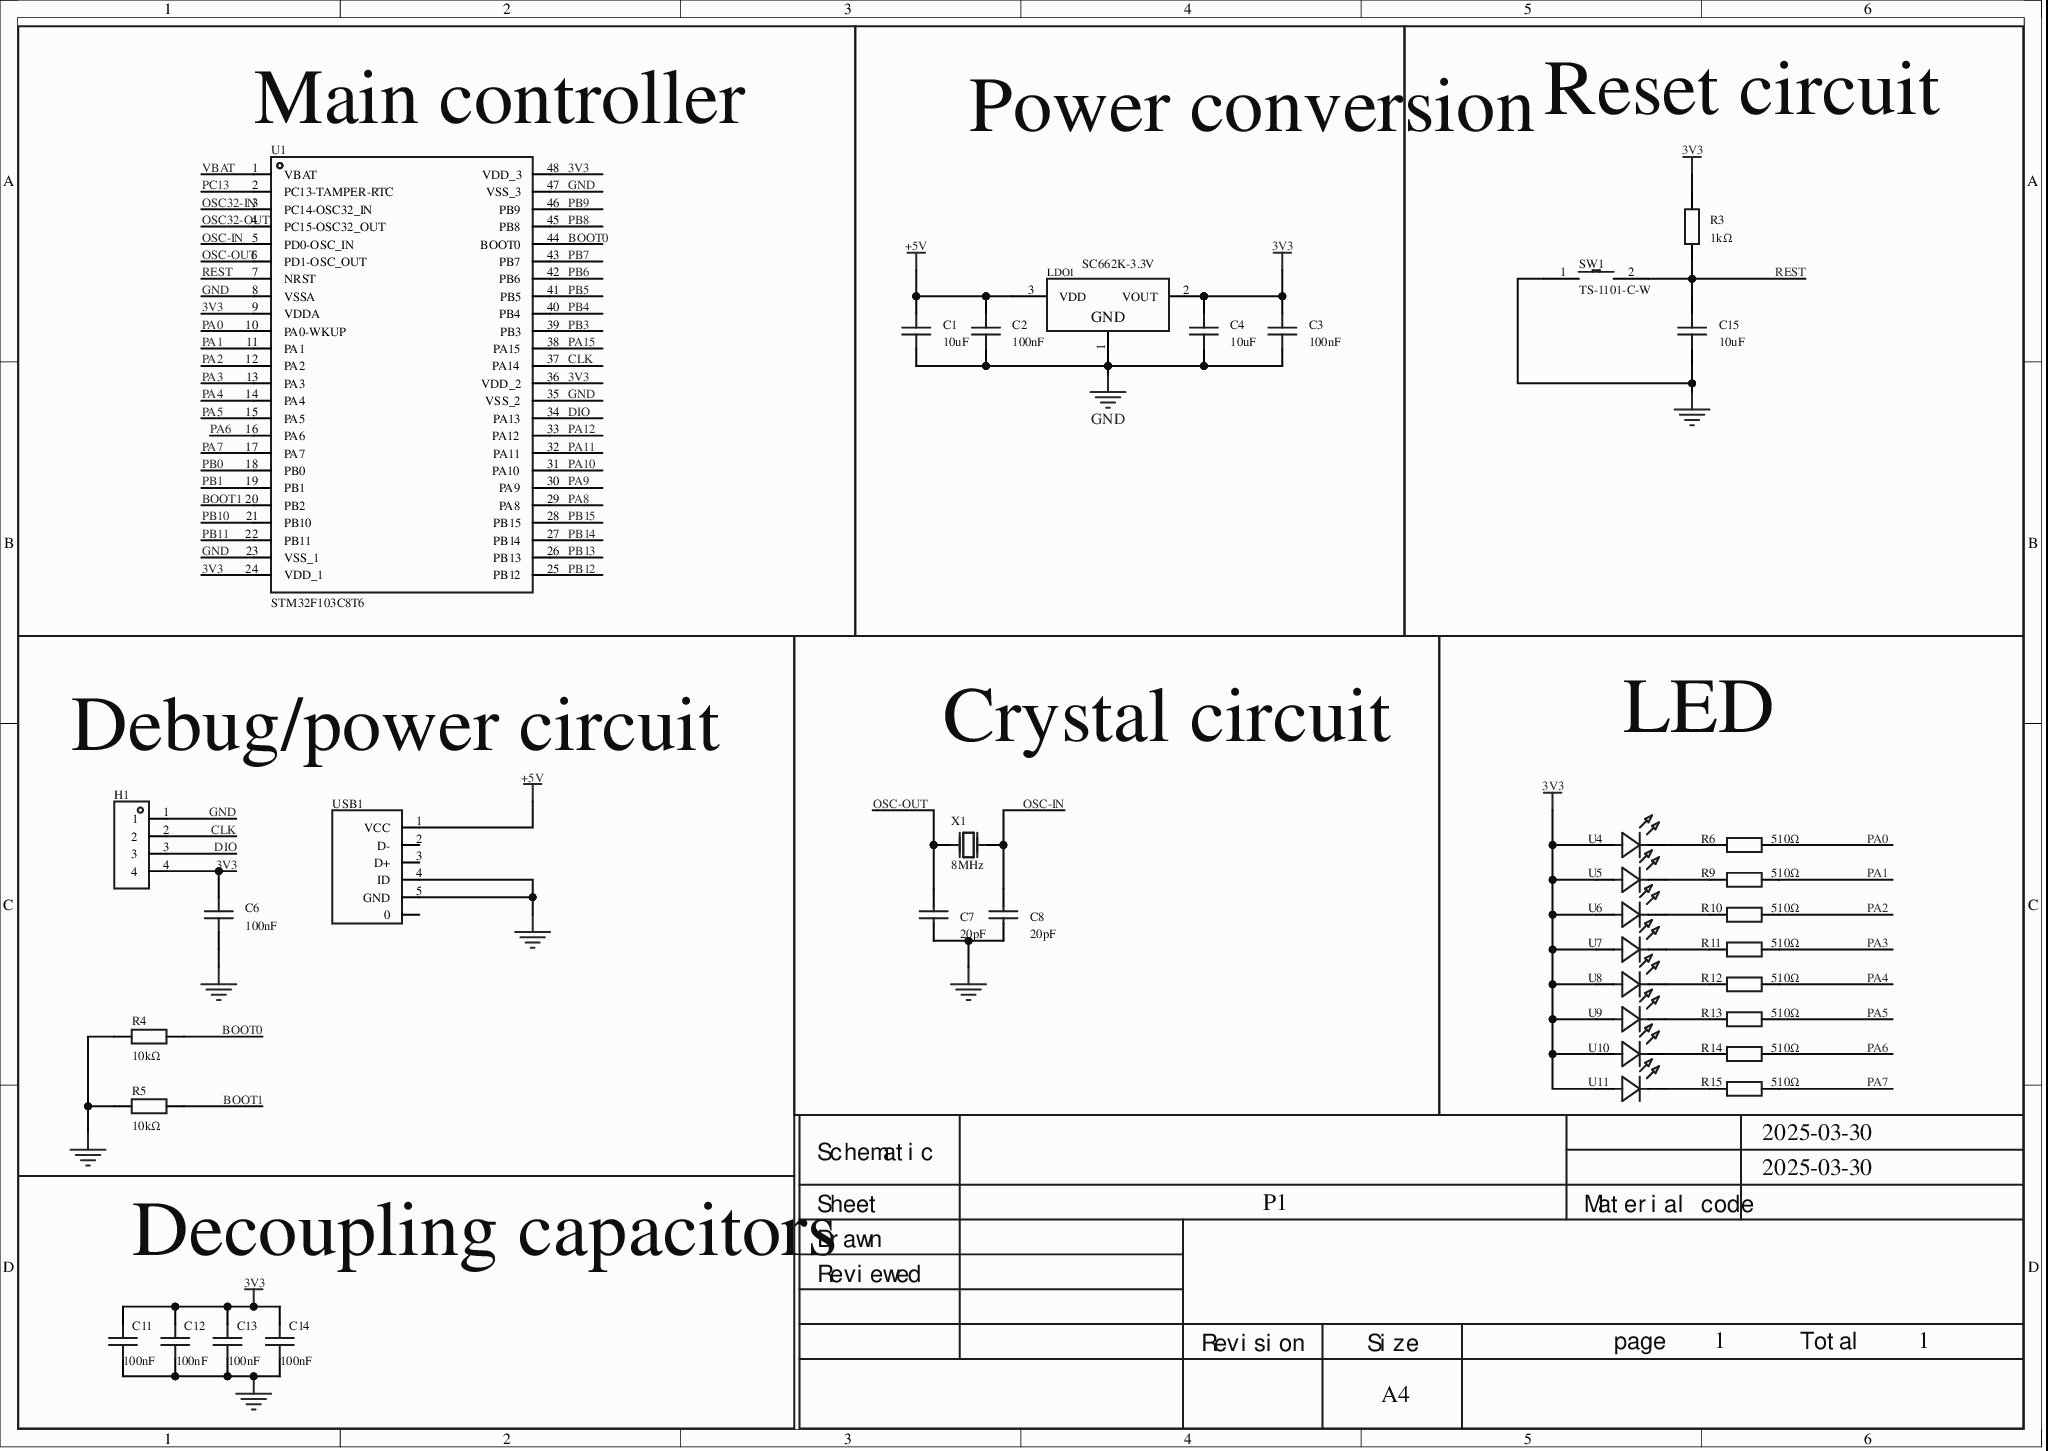
[diagram p0: MISC61263-3.schdoc]
# Altium project MISC61263-2.PrjPcb
1 sheet, 37 parts. Net scope: global (net labels, ports and power ports of the same name join across sheets).
Board file: MISC61263.pcbdoc

## Sheet MISC61263-3.schdoc
size 297 x 210 mm; Version: V1.0; @Project Name: MISC61263; @Page Count: 1; @Update Date: 2025-03-30; @Create Date: 2025-03-30; @Schematic Name: MISC61263; @Page No: 1; @Board Name: MISC61263; @Create Time: 16:09:01; @Update Time: 17:01:16

### Parts
C1  10uF  [C0603]
C2  100nF  [C0603]
C3  100nF  [C0603]
C4  10uF  [C0603]
C6  100nF  [C0603]
C7  20pF  [C0603]
C8  20pF  [C0603]
C11  100nF  [C0603]
C12  100nF  [C0603]
C13  100nF  [C0603]
C14  100nF  [C0603]
C15  10uF  [C0603]
H1  (no value)  [HDR-TH_4P-P2.54-V-M]
LDO1  SC662K-3.3V  [SOT-23-3_L2.9-W1.3-P1.90-LS2.4-BR]
R3  1kΩ  [R0603]
R4  10kΩ  [R0603]
R5  10kΩ  [R0603]
R6  510Ω  [R0603]
R9  510Ω  [R0603]
R10  510Ω  [R0603]
R11  510Ω  [R0603]
R12  510Ω  [R0603]
R13  510Ω  [R0603]
R14  510Ω  [R0603]
R15  510Ω  [R0603]
SW1  TS-1101-C-W  [SW-SMD_L6.0-W3.3-LS8.0]
U1  STM32F103C8T6  [LQFP-48_L7.0-W7.0-P0.50-LS9.0-BL]
U4  42-51/GHC-YW2X2K/3T  [LED-SMD_L1.6-W0.8-FD_GREEN-1]  (value not drawn)
U5  42-51/GHC-YW2X2K/3T  [LED-SMD_L1.6-W0.8-FD_GREEN-1]  (value not drawn)
U6  42-51/GHC-YW2X2K/3T  [LED-SMD_L1.6-W0.8-FD_GREEN-1]  (value not drawn)
U7  42-51/GHC-YW2X2K/3T  [LED-SMD_L1.6-W0.8-FD_GREEN-1]  (value not drawn)
U8  42-51/GHC-YW2X2K/3T  [LED-SMD_L1.6-W0.8-FD_GREEN-1]  (value not drawn)
U9  42-51/GHC-YW2X2K/3T  [LED-SMD_L1.6-W0.8-FD_GREEN-1]  (value not drawn)
U10  42-51/GHC-YW2X2K/3T  [LED-SMD_L1.6-W0.8-FD_GREEN-1]  (value not drawn)
U11  42-51/GHC-YW2X2K/3T  [LED-SMD_L1.6-W0.8-FD_GREEN-1]  (value not drawn)
USB1  920-D62A2021S10100  [MICRO-USB-SMD_5P-P0.65-H-M_MICRO-USB-5P]  (value not drawn)
X1  8MHz  [OSC-TH_L10.0-W4.5-P5.00]

### Blocks framed on the sheet
Main controller: U1
Power conversion: C1-C4 LDO1
Reset circuit: C15 R3 SW1
Debug/power circuit: C6 H1 R4 R5 USB1
Crystal circuit: C7 C8 X1
LED: R6 R9-R15 U4-U11
Decoupling capacitors: C11-C14

### Nets
3V3: C3.2 C4.2 C6.2 C11.2 C12.2 C13.2 C14.2 H1.4 LDO1.2(VOUT) R3.2 U1.9(VDDA) U1.24(VDD_1) U1.36(VDD_2) U1.48(VDD_3) U4.1(A) U5.1(A) U6.1(A) U7.1(A) U8.1(A) U9.1(A) U10.1(A) U11.1(A)
+5V: C1.2 C2.2 LDO1.3(VDD) USB1.1(VCC)
GND: C1.1 C2.1 C3.1 C4.1 C6.1 C7.1 C8.1 C11.1 C12.1 C13.1 C14.1 C15.1 H1.1 LDO1.1(GND) R4.1 R5.1 SW1.1 U1.8(VSSA) U1.23(VSS_1) U1.35(VSS_2) U1.47(VSS_3) USB1.4(ID) USB1.5(GND)
BOOT0: R4.2 U1.44(BOOT0)
BOOT1: R5.2 U1.20(PB2)
CLK: H1.2 U1.37(PA14)
DIO: H1.3 U1.34(PA13)
OSC32-IN: U1.3(PC14-OSC32_IN)
OSC32-OUT: U1.4(PC15-OSC32_OUT)
OSC-IN: C8.2 U1.5(PD0-OSC_IN) X1.1(OSC1)
OSC-OUT: C7.2 U1.6(PD1-OSC_OUT) X1.2(OSC2)
PA0: R6.2 U1.10(PA0-WKUP)
PA1: R9.2 U1.11(PA1)
PA2: R10.2 U1.12(PA2)
PA3: R11.2 U1.13(PA3)
PA4: R12.2 U1.14(PA4)
PA5: R13.2 U1.15(PA5)
PA6: R14.2 U1.16(PA6)
PA7: R15.2 U1.17(PA7)
PA8: U1.29(PA8)
PA9: U1.30(PA9)
PA10: U1.31(PA10)
PA11: U1.32(PA11)
PA12: U1.33(PA12)
PA15: U1.38(PA15)
PB0: U1.18(PB0)
PB1: U1.19(PB1)
PB3: U1.39(PB3)
PB4: U1.40(PB4)
PB5: U1.41(PB5)
PB6: U1.42(PB6)
PB7: U1.43(PB7)
PB8: U1.45(PB8)
PB9: U1.46(PB9)
PB10: U1.21(PB10)
PB11: U1.22(PB11)
PB12: U1.25(PB12)
PB13: U1.26(PB13)
PB14: U1.27(PB14)
PB15: U1.28(PB15)
PC13: U1.2(PC13-TAMPER-RTC)
REST: C15.2 R3.1 SW1.2 U1.7(NRST)
VBAT: U1.1(VBAT)
NetR6_1: R6.1 U4.2(C)
NetR9_1: R9.1 U5.2(C)
NetR10_1: R10.1 U6.2(C)
NetR11_1: R11.1 U7.2(C)
NetR12_1: R12.1 U8.2(C)
NetR13_1: R13.1 U9.2(C)
NetR14_1: R14.1 U10.2(C)
NetR15_1: R15.1 U11.2(C)

Not connected (* = marked no-connect by the designer): USB1 0* 2(D-) 3(D+)

### Notes on the sheet
- 2025-03-30
- Schematic
- Sheet
- P1
- Material code
- Reviewed
- Drawn
- Revision
- Size
- A4
- page
- 1
- Total

### Library data of the parts
C1 C4 C15 = CL10A106KP8NNNC: Capacitance: 10uF; tolerance: ±10%; rated voltage: 10V; dielectric (temperature coefficient): X5R;; Manufacturer: SAMSUNG(三星); AddInBom: yes; ModelId: ac125912035d415993ca9572d50418b1; ModelName: C0603_L1.6-W0.8-H0.8; ModelTransform: 62.992,31.496,0,0,0,0,0,0,0; Device: CL10A106KP8NNNC; Symbol: CL10A106KP8NNNC; LCSC Part Name: 10uF ±10% 10V; SupplierPart: C19702; ManufacturerPart: CL10A106KP8NNNC; Supplier Footprint: 0603; JLCPCB Part Class: Basic library; Datasheet: https://atta.szlcsc.com/upload/public/pdf/source/20160103/1457707703378.pdf; Supplier: LCSC; ConvertToPcb: yes; FootprintName: C0603; Value: 10uF; Tolerance: ±10%; Voltage Rated: 10V; Temperature Coefficient: X5R
C2 C3 = CC0603KRX7R9BB104: Capacitance: 100nF; tolerance: ±10%; rated voltage: 50V; dielectric (temperature coefficient): X7R;; Manufacturer: YAGEO(国巨); AddInBom: yes; ModelId: ac125912035d415993ca9572d50418b1; ModelName: C0603_L1.6-W0.8-H0.8; ModelTransform: 62.992,31.496,0,0,0,0,0,0,0; Device: CC0603KRX7R9BB104; Symbol: CC0603KRX7R9BB104; LCSC Part Name: 100nF ±10% 50V; SupplierPart: C14663; ManufacturerPart: CC0603KRX7R9BB104; Supplier Footprint: 0603; JLCPCB Part Class: Basic library; Datasheet: https://atta.szlcsc.com/upload/public/pdf/source/20180910/C282072_33301C7F631E79921B82A8DAC6BCC5B3.pdf; Supplier: LCSC; ConvertToPcb: yes; FootprintName: C0603; Value: 100nF; Tolerance: ±10%; Voltage Rated: 50V; Temperature Coefficient: X7R
C6 C11-C14 = CGA0603X7R104K500JT: Capacitance: 100nF; tolerance: ±10%; rated voltage: 50V; dielectric (temperature coefficient): X7R;; Manufacturer: HRE(芯声); AddInBom: yes; ModelId: ac125912035d415993ca9572d50418b1; ModelName: C0603_L1.6-W0.8-H0.8; ModelTransform: 62.992,31.496,0,0,0,0,0,0,0; Symbol: CGA0603X7R104K500JT; Device: CGA0603X7R104K500JT; LCSC Part Name: 100nF ±10% 50V; SupplierPart: C6119867; ManufacturerPart: CGA0603X7R104K500JT; Supplier Footprint: 0603; JLCPCB Part Class: Extended library; Supplier: LCSC; ConvertToPcb: yes; FootprintName: C0603; Value: 100nF; Tolerance: ±10%; Voltage Rated: 50V; Temperature Coefficient: X7R
C7 C8 = CL10C200JB8NNNC: Capacitance: 20pF; tolerance: ±5%; rated voltage: 50V; dielectric (temperature coefficient): C0G;; Manufacturer: SAMSUNG(三星); AddInBom: yes; ModelId: ac125912035d415993ca9572d50418b1; ModelName: C0603_L1.6-W0.8-H0.8; ModelTransform: 62.992,31.496,0,0,0,0,0,0,0; Symbol: CL10C200JB8NNNC; Device: CL10C200JB8NNNC; LCSC Part Name: 20pF ±5% 50V; SupplierPart: C1648; ManufacturerPart: CL10C200JB8NNNC; Supplier Footprint: 0603; JLCPCB Part Class: Basic library; Datasheet: https://atta.szlcsc.com/upload/public/pdf/source/20160218/1457707763339.pdf; Supplier: LCSC; ConvertToPcb: yes; FootprintName: C0603; Value: 20pF; Tolerance: ±5%; Voltage Rated: 50V; Temperature Coefficient: C0G
H1 = HDR-M_2.54_1x4P: Symbol: PZ254V-11-04P; ConvertToPcb: yes; ModelId: 112f4d05e8d64e99ab9a333894bea4f9; ModelName: HDR-TH_4P-P2.54-M-LI-1X4P; ModelTransform: 399.999,104.7242,0,0,0,0,0,0,-118.11; Device: HDR-M_2.54_1x4P; AddInBom: yes; SupplierPart: C492403; Supplier Footprint: 插件; FootprintName: HDR-TH_4P-P2.54-V-M
LDO1 = SC662K-3.3V: Output type: fixed; output polarity: positive; max input voltage: 6V; output voltage: 3.3V; output current: 250mA; power supply ripple rejection (PSRR): 50dB@(1kHz);; Manufacturer: FM(富满); AddInBom: yes; ModelId: c62791f0466c4ae2a892c056b845b0ca; ModelName: SOT-23-3P_L2.9-W1.3-H1.0-LS2.4-P0.95; ModelTransform: 98.425,114.173,0,180,0,0,0.0005,-0.0005,0; Number of Outputs: 1; Dropout Voltage: 38mV@(10mA); Symbol: SC662K-3.3V; Device: SC662K-3.3V; Supplier: LCSC; Manufacturer Part: SC662K-3.3V; Supplier Part: C83932; JLCPCB Part Class: Extended library; LCSC Part Name: 输入6V 输出3.3V 250mA 停产; Supplier Footprint: SOT-23; Datasheet: https://atta.szlcsc.com/upload/public/pdf/source/20161024/1477288576049.pdf; ConvertToPcb: yes; FootprintName: SOT-23-3_L2.9-W1.3-P1.90-LS2.4-BR; Output Type: Fixed; Output Polarity: Positive; Maximum Input Voltage: 6V; Output Voltage: 3.3V; Output Current: 250mA; Power Supply Rejection Ratio (PSRR): 50dB@(1kHz)
R3 = RC0603FR-071KL: Resistor type: thick film resistor; resistance: 1kΩ; tolerance: ±1%; power: 100mW; max working voltage: 75V; temperature coefficient: ±100ppm/℃;; Manufacturer: YAGEO(国巨); AddInBom: yes; ModelId: fc143cca1e79419f9cd78b61e9279f08; ModelTransform: 31.8897,63.7794,0,90,0,0,0,0,0; Symbol: RC0603FR-071KL; Device: RC0603FR-071KL; LCSC Part Name: 厚膜电阻 1kΩ ±1% 100mW; SupplierPart: C22548; ManufacturerPart: RC0603FR-071KL; Supplier Footprint: 0603; JLCPCB Part Class: Extended library; Datasheet: https://atta.szlcsc.com/upload/public/pdf/source/20180316/70C0E2BDAE7FCC62C531A5A58D202EE1.pdf; Supplier: LCSC; ConvertToPcb: yes; FootprintName: R0603; ModelName: R0603; Type: Thick film resistor; Value: 1kΩ; Tolerance: ±1%; Power(Watts): 100mW; Overload Voltage (Max): 75V; Temperature Coefficient: ±100ppm/℃; Operating Temperature Range: -55℃~+155℃
R4 R5 = 0603WAF1002T5E: Resistor type: thick film resistor; resistance: 10kΩ; tolerance: ±1%; power: 100mW; max working voltage: 75V; temperature coefficient: ±100ppm/℃;; Manufacturer: UNI-ROYAL(厚声); AddInBom: yes; ModelId: fc143cca1e79419f9cd78b61e9279f08; ModelTransform: 31.8897,63.7794,0,90,0,0,0,0,0; Symbol: 0603WAF1002T5E; Device: 0603WAF1002T5E; LCSC Part Name: 厚膜电阻 10kΩ ±1% 100mW; SupplierPart: C25804; ManufacturerPart: 0603WAF1002T5E; Supplier Footprint: 0603; JLCPCB Part Class: Basic library; Datasheet: https://atta.szlcsc.com/upload/public/pdf/source/20200306/C422600_1E6D84923E4A46A82E41ADD87F860B5C.pdf; Supplier: LCSC; ConvertToPcb: yes; FootprintName: R0603; ModelName: R0603; Type: Thick film resistor; Value: 10kΩ; Tolerance: ±1%; Power(Watts): 100mW; Overload Voltage (Max): 75V; Temperature Coefficient: ±100ppm/℃; Operating Temperature Range: -55℃~+155℃
R6 R9-R15 = 0603WAF5100T5E: Resistor type: thick film resistor; resistance: 510Ω; tolerance: ±1%; power: 100mW; max working voltage: 75V; temperature coefficient: ±100ppm/℃;; Manufacturer: UNI-ROYAL(厚声); AddInBom: yes; ModelId: fc143cca1e79419f9cd78b61e9279f08; ModelTransform: 31.8897,63.7794,0,90,0,0,0,0,0; Symbol: 0603WAF5100T5E; Device: 0603WAF5100T5E; LCSC Part Name: 510Ω ±1% 100mW 厚膜电阻; SupplierPart: C23193; ManufacturerPart: 0603WAF5100T5E; Supplier Footprint: 0603; JLCPCB Part Class: Basic library; Datasheet: https://atta.szlcsc.com/upload/public/pdf/source/20200306/C422600_1E6D84923E4A46A82E41ADD87F860B5C.pdf; Supplier: LCSC; ConvertToPcb: yes; FootprintName: R0603; ModelName: R0603; Type: Thick film resistor; Value: 510Ω; Tolerance: ±1%; Power(Watts): 100mW; Overload Voltage (Max): 75V; Temperature Coefficient: ±100ppm/℃; Operating Temperature Range: -55℃~+155℃
SW1 = TS-1101-C-W: Circuit structure: SPST; button shape: rectangular button; actuation force: 260gf; mounting: upright SMD; switch length: 6mm; switch width: 3.6mm; switch height: 2.5mm; with bracket: without; contact current: 50mA; rated voltage (AC): -; rated voltage (DC): 12V; rated power: -; insulation resistance: -; with lamp: none; mechanical life: 5万 cycles;; Manufacturer: XKB Connectivity(中国星坤); AddInBom: yes; ModelId: b2f4ea9f0afc4b0786d53dba66ceb9e4; ModelName: SW-SMD_L6.0-W3.3-H5-LS8.0; ModelTransform: 314.96,129.921,0,0,0,0,0,0,0; Actuator/Cap Color: White with light green tint; Symbol: TS-1101-C-W; Device: TS-1101-C-W; LCSC Part Name: 6*3.6*2.5mm 立贴 轻触开关; SupplierPart: C318938; ManufacturerPart: TS-1101-C-W; Supplier Footprint: SMD; JLCPCB Part Class: Extended library; Datasheet: https://atta.szlcsc.com/upload/public/pdf/source/20200227/C318938_C2E53B1EEDE37D980A33616AC086DE53.pdf; Supplier: LCSC; ConvertToPcb: yes; FootprintName: SW-SMD_L6.0-W3.3-LS8.0; Circuit: SPST; Actuator Style: Rectangular button; Operating Force: 260gf; Mounting Style: Upright SMD; Switch Length: 6mm; Switch Width: 3.6mm; Switch Height: 2.5mm; Strike Gundam: Without; Contact Current: 50mA; Voltage Rating (AC): -; Voltage Rating (DC): 12V; Power Rating: -; Insulation Resistance: -; With Lamp: None; IP Rating: -; Pin Style: -; Mechanical Life: 5万 cycles; Operating Temperature: -30℃~+85℃
U1 = STM32F103C8T6: CPU core: ARM-M3; program storage capacity: 64KB; RAM total: 20KB; GPIO port count: 37; operating voltage range: 2V~3.6V; max CPU frequency: 72MHz; program memory type: FLASH;; Manufacturer: ST(意法半导体); AddInBom: yes; ModelId: 093be70396ff421eb2cdb946d5311efc; ModelName: LQFP-48_L7.0-W7.0-H1.4-LS9.0-P0.50; ModelTransform: 354.331,354.331,0,0,0,0,0,0,0; GPIO Ports Number: 37; ADC (Bit): 12bit; Peripheral/Function: Watchdog; DMA; watchdog; temperature sensor; Symbol: STM32F103C8T6; Device: STM32F103C8T6; LCSC Part Name: 主流增强型ARM Cortex-M3 MCU，具有64 KB Flash、72 MHz CPU、电机控制、USB和CAN; SupplierPart: C8734; ManufacturerPart: STM32F103C8T6; Supplier Footprint: LQFP-48(7x7); JLCPCB Part Class: Extended library; Datasheet: https://atta.szlcsc.com/upload/public/pdf/source/20220812/8363ACEC51AD55ECEB84799464F7CB85.pdf; Supplier: LCSC; ConvertToPcb: yes; FootprintName: LQFP-48_L7.0-W7.0-P0.50-LS9.0-BL; CPU Core: ARM-M3; Program Storage Size: 64KB; RAM Size: 20KB; Operating Voltage Range: 2V~3.6V; CPU Maximum Speed: 72MHz; Program Memory Type: FLASH; Operating Temperature Range: -40℃~+85℃; DAC (Bit): -; PWM (Bit): -; Universal Serial Bus: Yes; Internal Comparator: -; communication protocol: -; Watchdog: Yes; Real-Time Clock: -; Infrared Data Association: Yes; Low-Voltage Detect: Yes; CCP Capture/Compare: -; Secure Digital Input and Output: -; Direct Memory Access: Yes; Internal Oscillator: Yes
U4-U11 = 42-51/GHC-YW2X2K/3T: Emitted color: emerald green; forward current: -; dominant wavelength: 520nm~535nm; luminous intensity: 2850mcd;; Manufacturer: EVERLIGHT(亿光); AddInBom: yes; ModelId: feee2acead2344579596fed70e7e7f0f; ModelTransform: 63.7794,31.89954,0,0,0,0,0,0,0; Symbol: 42-51/GHC-YW2X2K/3T; Device: 42-51/GHC-YW2X2K/3T; LCSC Part Name: 正发光贴片灯 颜色正绿色 发光二极管; SupplierPart: C5136797; ManufacturerPart: 42-51/GHC-YW2X2K/3T; Supplier Footprint: 0603; JLCPCB Part Class: Extended library; Datasheet: https://atta.szlcsc.com/upload/public/pdf/source/20220916/FBE88CF67A3FC292A254CF6ACE30EBDE.pdf; Supplier: LCSC; ConvertToPcb: yes; FootprintName: LED-SMD_L1.6-W0.8-FD_GREEN-1; ModelName: LED-SMD_L1.6-W0.8-FD_GREEN-1; Emitted Color: Emerald green; Forward Current: -; Dominant Wavelength: 520nm~535nm; Luminous Intensity: 2850mcd
USB1 = 920-D62A2021S10100: Connector type: Micro-B; standard: USB 2.0; gender: female; contacts: 5P; ports: 1; rated current - power: 1A;; Manufacturer: 精拓金; Symbol: Micro USB-B 5P_C40942; AddInBom: yes; ModelId: 81679493ca6f46a8bef4e1c4a07d5303; ModelTransform: 307.086,217.126,0,180,0,0,0,-32.679,-23.622; Number of Ports: 1; Device: 920-D62A2021S10100; Supplier: LCSC; Manufacturer Part: 920-D62A2021S10100; Supplier Part: C40942; JLCPCB Part Class: Extended library; LCSC Part Name: Micro-B 母; Supplier Footprint: SMD; Datasheet: https://atta.szlcsc.com/upload/public/pdf/source/20210308/C40942_64F4AC38F8216E0A4EC315319D07B0C5.pdf; ConvertToPcb: yes; FootprintName: MICRO-USB-SMD_5P-P0.65-H-M_MICRO-USB-5P; ModelName: MICRO-USB-SMD_5P-P0.65-H-M_MICRO-USB-5P; Connector Type: Micro-B; Standard: USB 2.0; Gender: Female; Number of Contacts: 5P; Current Rating - Power (Max): 1A
X1 = X49SD8MSD2SC: Crystal type: through-hole crystal; frequency: 8MHz; frequency tolerance at room temperature: ±20ppm; external load capacitance: 20pF; frequency stability (full temperature): ±30ppm;; Manufacturer: YXC(扬兴晶振); AddInBom: yes; ModelId: a8e34f6c394c4d60ace7720f62d1ccdf; ModelName: HC-49US_L11.0-W4.5-H3.5-P4.88; ModelTransform: 432.46488,177.165,0,90,0,0,0,0,-137.795; Symbol: X49SD8MSD2SC; Device: X49SD8MSD2SC; LCSC Part Name: 8MHz ±20ppm 20pF; SupplierPart: C21263; ManufacturerPart: X49SD8MSD2SC; Supplier Footprint: HC-49S; JLCPCB Part Class: Extended library; Datasheet: https://atta.szlcsc.com/upload/public/pdf/source/20240329/977D7F2434F98B2BE33270BB9FF3D86D.pdf; Supplier: LCSC; ConvertToPcb: yes; FootprintName: OSC-TH_L10.0-W4.5-P5.00; Crystal Type: Through-hole crystal; Value: 8MHz; Normal temperature Frequency Tolerance: ±20ppm; External load capacitor: 20pF; Frequency Stability(Full temperature range): ±30ppm; Operating Temperature: -20℃~+70℃